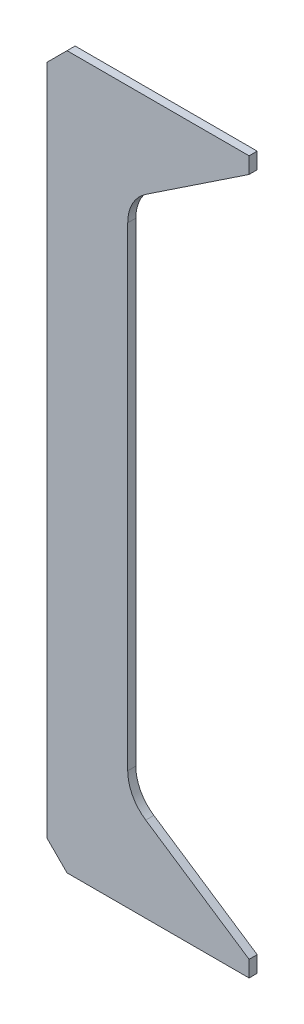
from build123d import *

# Parameters (mm, degrees)
SKETCH1_W           = 150
SKETCH1_H           = 20
SKETCH1_W_2         = 100
BOSS_EXTRUDE1_DEPTH = 10
FILLET1_R           = 50
CHAMFER1_SIZE       = 25


with BuildPart() as part:
    # Sketch1 → Boss-Extrude1 (new body)
    with BuildSketch(Plane.XY):
        Polygon((200, 420), (50, 420), (50, 320), align=None)
        with Locations((125, 430)):
            Rectangle(SKETCH1_W, SKETCH1_H)
        Polygon((-50, 420), (-50, -420), (50, -420), (50, -320), (50, 320), (50, 420), align=None)
        Polygon((50, -320), (50, -420), (200, -420), align=None)
        with Locations((125, -430)):
            Rectangle(SKETCH1_W, SKETCH1_H)
        with Locations((0, -430)):
            Rectangle(SKETCH1_W_2, SKETCH1_H)
        with Locations((0, 430)):
            Rectangle(SKETCH1_W_2, SKETCH1_H)
    extrude(amount=BOSS_EXTRUDE1_DEPTH)

    # Fillet1
    fillet1_edges = [part.edges().sort_by_distance(p)[0] for p in [
        (50, 320, 5),
        (50, -320, 5),
    ]]
    fillet(fillet1_edges, radius=FILLET1_R)

    # Chamfer1
    chamfer1_edges = [part.edges().sort_by_distance(p)[0] for p in [
        (-50, -440, 5),
        (-50, 440, 5),
    ]]
    chamfer(chamfer1_edges, length=CHAMFER1_SIZE)


solid = part.part
